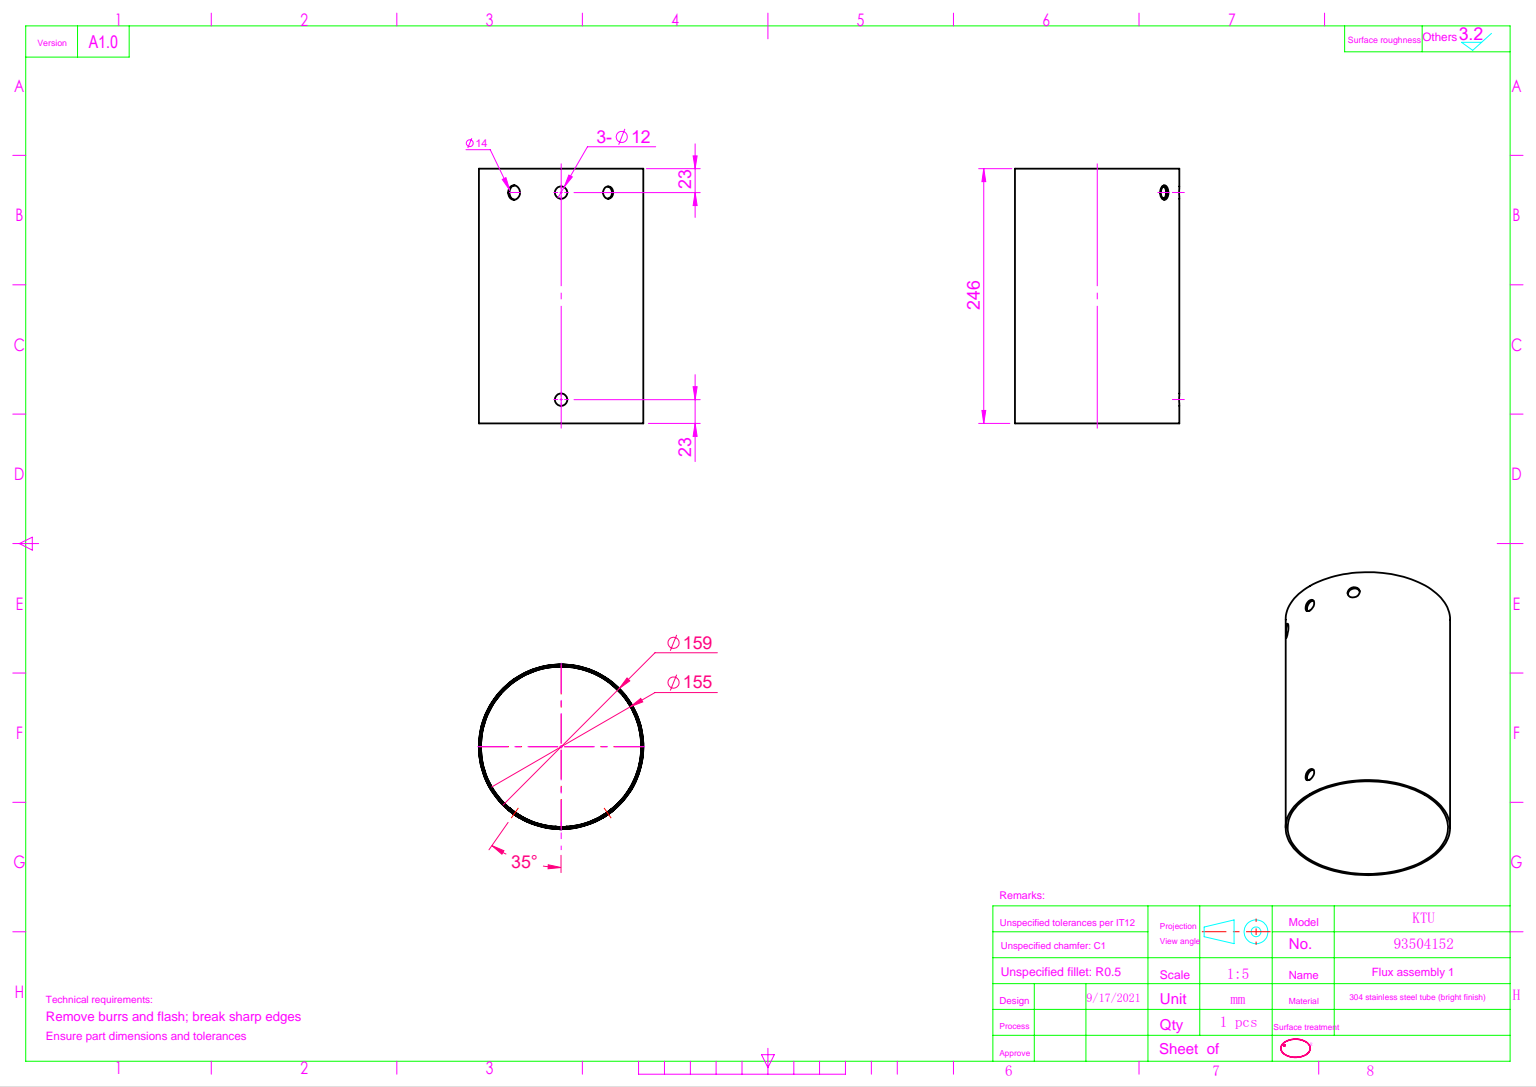
from build123d import *

# Parameters (mm, degrees)
SKETCH_2_R          = 79.5
SKETCH_2_R_2        = 77.5
EXTRUDE_1_DEPTH     = 123
SKETCH_3_R          = 6
CUT_EXTRUDE_2_DEPTH = 167.641831483
SKETCH_4_R          = 6
CUT_EXTRUDE_3_DEPTH = 167.641831653
SKETCH_5_R          = 7
CUT_EXTRUDE_4_DEPTH = 167.641831653


with BuildPart() as part:
    # 草图2 → 拉伸-薄壁1 (new, symmetric)
    with BuildSketch(Plane(origin=(0, 0, 0), x_dir=(1, 0, 0), z_dir=(0, 1, 0))):
        Circle(SKETCH_2_R)
        Circle(SKETCH_2_R_2, mode=Mode.SUBTRACT)
    extrude(amount=EXTRUDE_1_DEPTH, both=True)

    # 草图3 → 切除-拉伸2 (cut, through all)
    with BuildSketch(Plane.XY):
        with Locations(Location((0, 100, 0), (0, 0, 180))):
            Circle(SKETCH_3_R)
        with Locations(Location((0, -100, 0), (0, 0, 180))):
            Circle(SKETCH_3_R)
    extrude(amount=CUT_EXTRUDE_2_DEPTH, mode=Mode.SUBTRACT)

    # 草图4 → 切除-拉伸3 (cut, through all)
    with BuildSketch(Plane(origin=(0, 0, 0), x_dir=(0, -1, 0), z_dir=(0.5735764363510444, 0, 0.819152044288993))):
        with Locations(Location((-100, 0, 0), (0, 0, 270))):
            Circle(SKETCH_4_R)
    extrude(amount=CUT_EXTRUDE_3_DEPTH, mode=Mode.SUBTRACT)

    # 草图5 → 切除-拉伸4 (cut, through all)
    with BuildSketch(Plane(origin=(0, 0, 0), x_dir=(0, -1, 0), z_dir=(0.5735764363510444, 0, -0.819152044288993))):
        with Locations(Location((-100, 0, 0), (0, 0, 90))):
            Circle(SKETCH_5_R)
    extrude(amount=-CUT_EXTRUDE_4_DEPTH, mode=Mode.SUBTRACT)


solid = part.part
